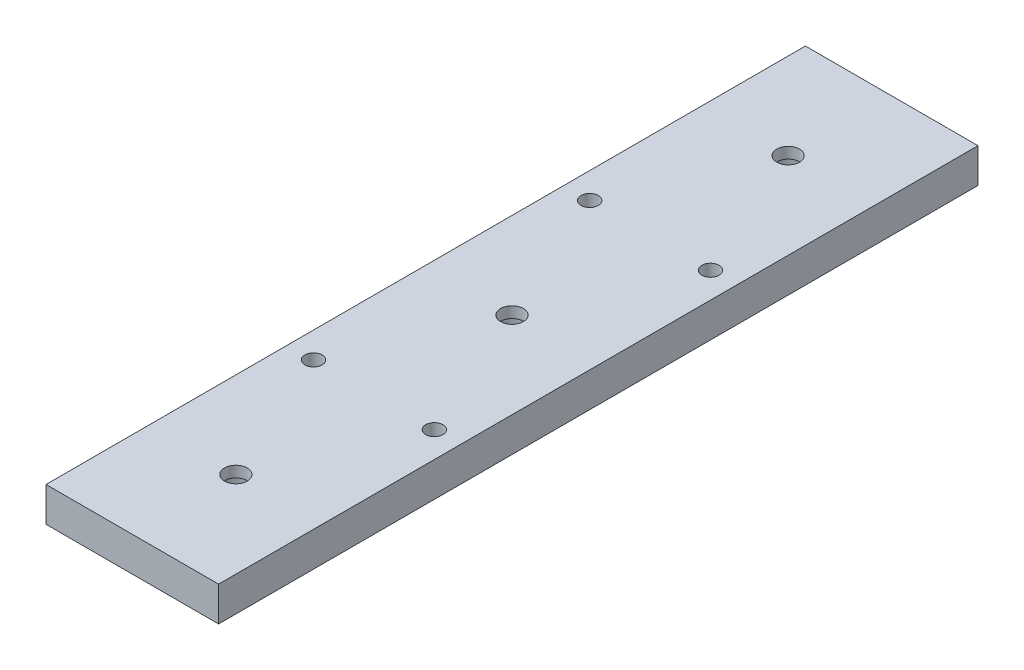
SolidWorks part; units mm, degrees
material "6061 Alloy"
ref_plane "Front Plane" through (0, 0, 0) normal (0, 0, 1) x (1, 0, 0)
ref_plane "Top Plane" through (0, 0, 0) normal (0, 1, 0) x (1, 0, 0)
ref_plane "Right Plane" through (0, 0, 0) normal (1, 0, 0) x (0, 0, -1)
sketch "Sketch1" plane through (0, 0, 0) normal (0, 1, 0) x (1, 0, 0)
  line L1 (-25, -110) -> (25, -110)
  line L2 (-25, -110) -> (-25, 110)
  line L3 (-25, 110) -> (25, 110)
  line L4 (25, -110) -> (25, 110)
  line L5 (-25, -110) -> (25, 110) construction
  line L6 (-25, 110) -> (25, -110) construction
  point P0 (0, 0)
  dimension "D1" = 220
  dimension "D2" = 50
extrude "Boss-Extrude1" add sketch "Sketch1" along normal blind 10
hole_wizard "Hole Size (% by) Socket Head Cap Screw Type1" positions "Sketch2" profile "Sketch4" counterbore size "M6" standard "GB" end condition through all
sketch "Sketch2" plane through (0, 0, 0) normal (0, -1, 0) x (-1, 0, 0)
  line L0 (0, -80) -> (0, 80) construction
  point P0 (0, -80)
  point P2 (0, 80)
  point P10 (0, 0)
  dimension "D1" = 160
sketch "Sketch4" plane through (0, 0, 80) normal (1, 0, 0) x (0, 0, -1)
  line L0 (0, 0) -> (0, 10)
  line L1 (0, 10) -> (3.3, 10)
  line L3 (3.3, 10) -> (3.3, 6.8)
  line L4 (3.3, 6.8) -> (5.5, 6.8)
  line L5 (5.5, 6.8) -> (5.5, 0)
  line L7 (5.5, 0) -> (0, 0)
  line L11 (0, -6.35) -> (0, 107.95) construction
  dimension "通孔孔直径" = 6.6
  dimension "通孔孔深度" = 10
  dimension "柱形沉头孔直径" = 11
  dimension "柱形沉头孔深度" = 6.8
hole_wizard "M6 Tapped Hole1" positions "Sketch5" profile "Sketch6" tap size "M6" standard "GB"
sketch "Sketch5" plane through (0, 10, 0) normal (0, 1, 0) x (1, 0, 0)
  line L0 (-17.5, 40) -> (-17.5, -40) construction
  line L1 (-17.5, 40) -> (17.5, 40) construction
  line L2 (17.5, 40) -> (17.5, -40) construction
  line L3 (17.5, -40) -> (-17.5, -40) construction
  line L6 (-17.5, 0) -> (0, 0) construction
  line L7 (0, 0) -> (0, 40) construction
  point P0 (-17.5, 40)
  point P2 (-17.5, -40)
  point P27 (17.5, 40)
  point P30 (17.5, -40)
  dimension "D1" = 80
  dimension "D2" = 35
sketch "Sketch6" plane through (-17.5, 10, -40) normal (1, 0, 0) x (0, 0, 1)
  line L0 (0, 0) -> (0, 16.5022)
  line L1 (0, 16.5022) -> (2.5, 15)
  line L2 (2.5, 15) -> (2.5, 0)
  line L5 (2.5, 0) -> (0, 0)
  line L10 (0, 16.5022) -> (-2.5, 15) construction
  line L11 (0, -6.35) -> (0, 107.95) construction
  dimension "螺纹孔钻头直径" = 5
  dimension "螺纹孔钻头深度" = 15
  dimension "导头角度" = 118
cosmetic thread "Hole Cosmetic Thread1" parameters "D1"=10, "D2"=6
cosmetic thread "Hole Cosmetic Thread2" parameters "D1"=10, "D2"=6
cosmetic thread "Hole Cosmetic Thread3" parameters "D1"=10, "D2"=6
cosmetic thread "Hole Cosmetic Thread4" parameters "D1"=10, "D2"=6
